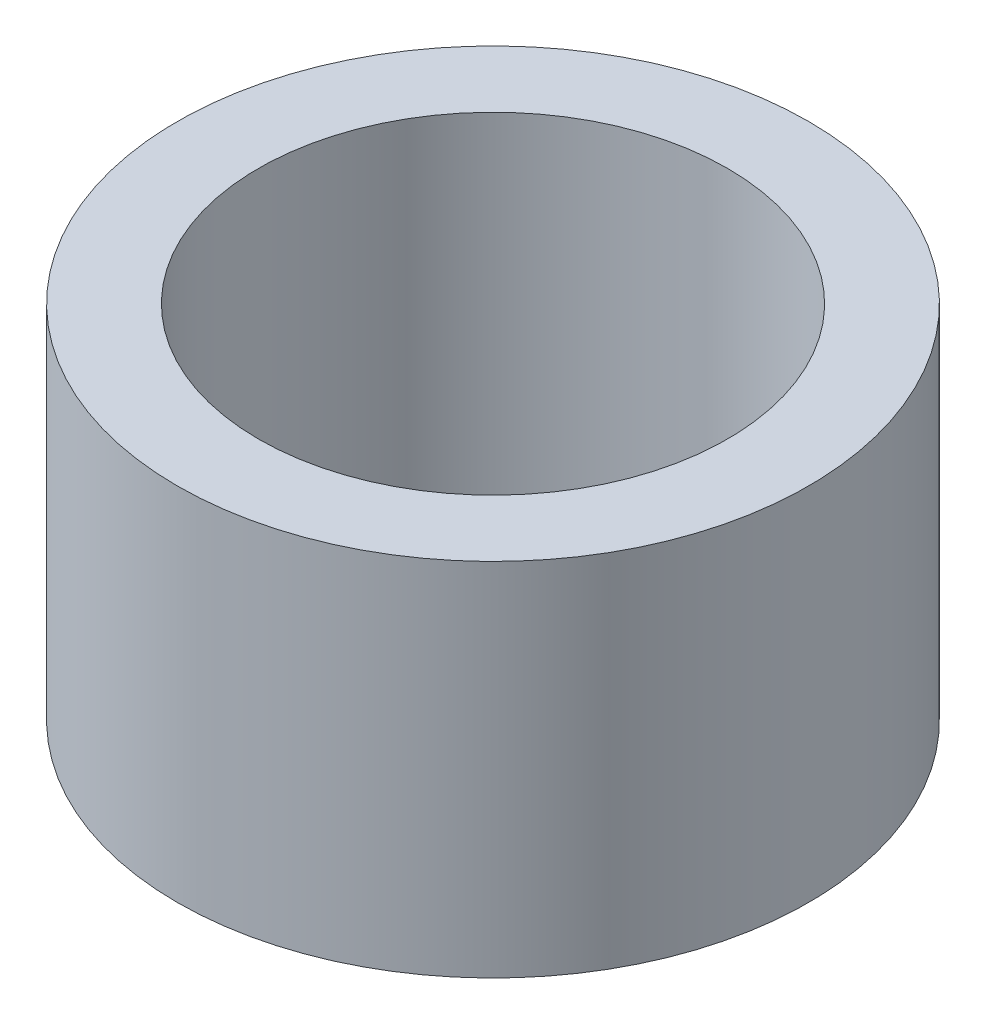
from build123d import *

# Parameters (mm, degrees)
SKETCH1_W = 4.5
SKETCH1_H = 20


with BuildPart() as part:
    # Sketch1 → Revolve1 (revolve)
    with BuildSketch(Plane.XY, mode=Mode.PRIVATE) as revolve1_sk:
        with Locations((-15.25, 4.181093582)):
            Rectangle(SKETCH1_W, SKETCH1_H)
    revolve(revolve1_sk.sketch.rotate(Axis((0, 22.656093582, 0), (0, -1, 0)), 270), axis=Axis((0, 22.656093582, 0), (0, -1, 0)))


solid = part.part
